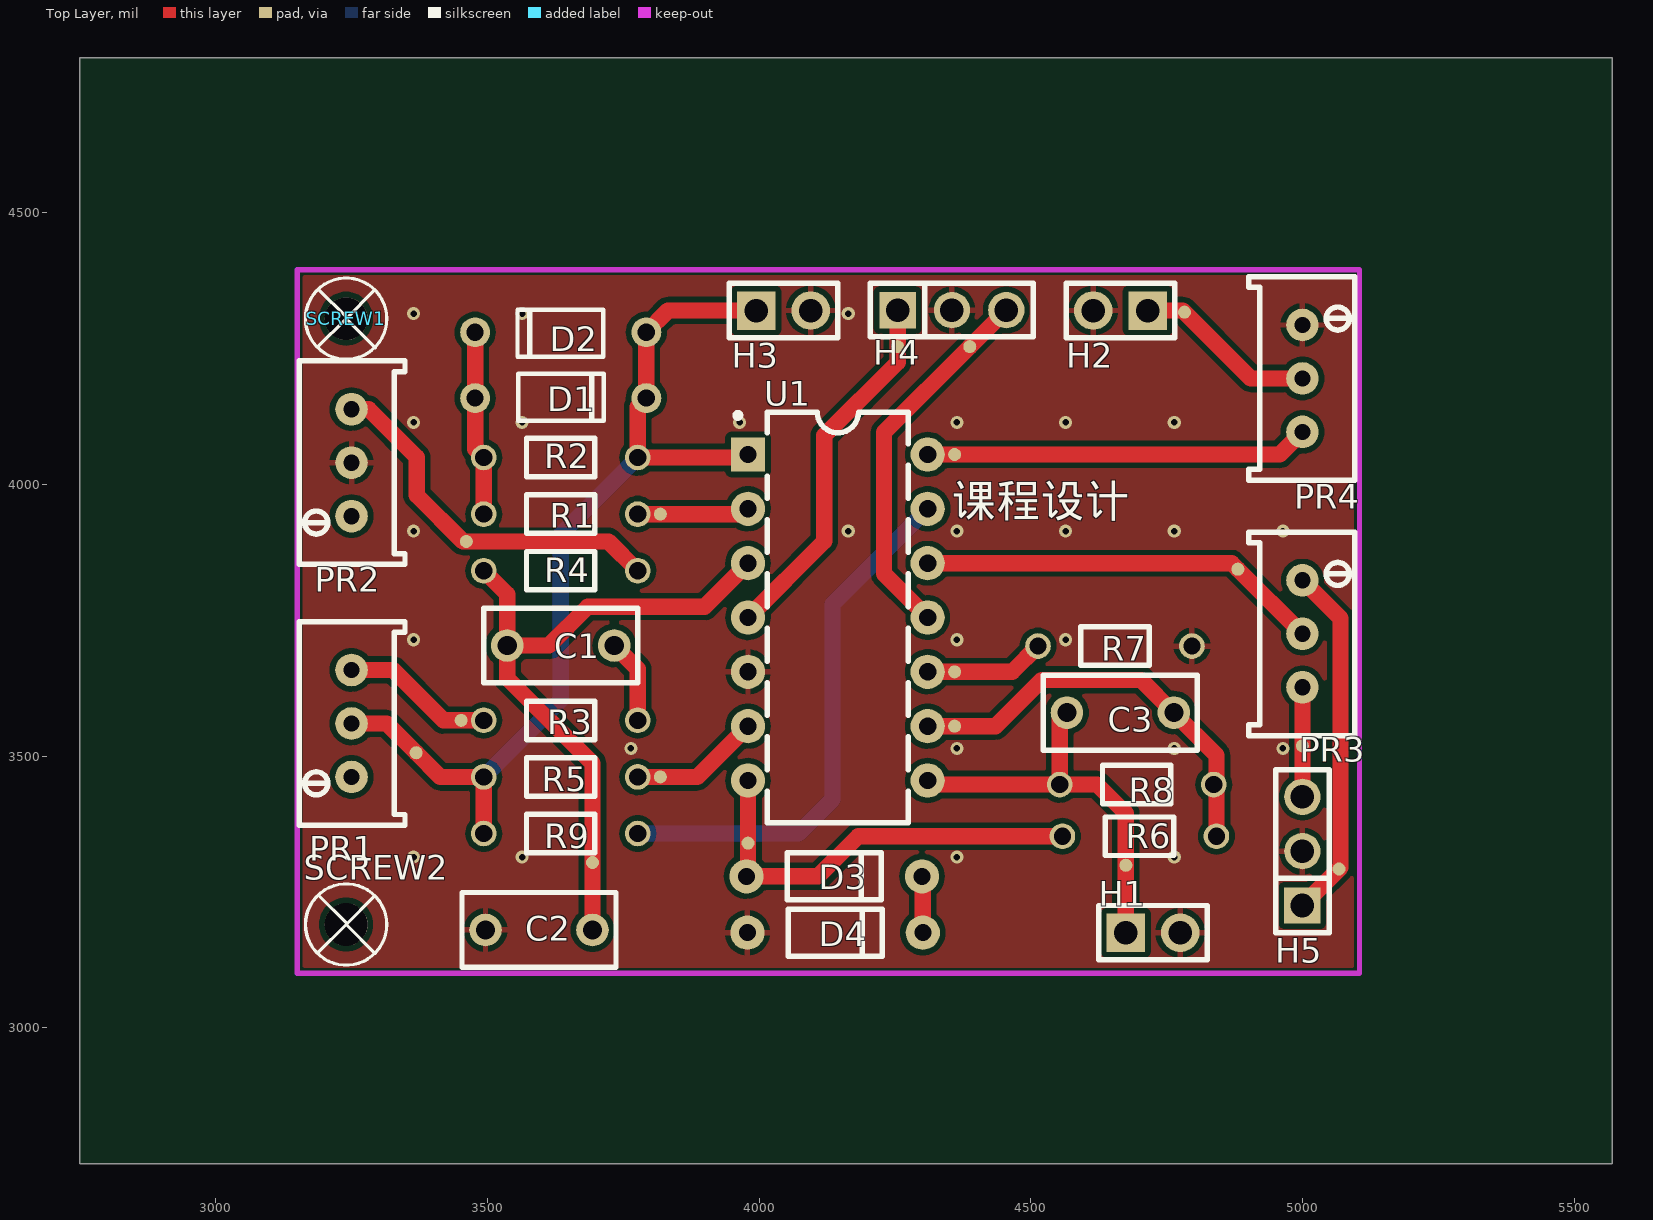
[diagram p0: Top Layer view]
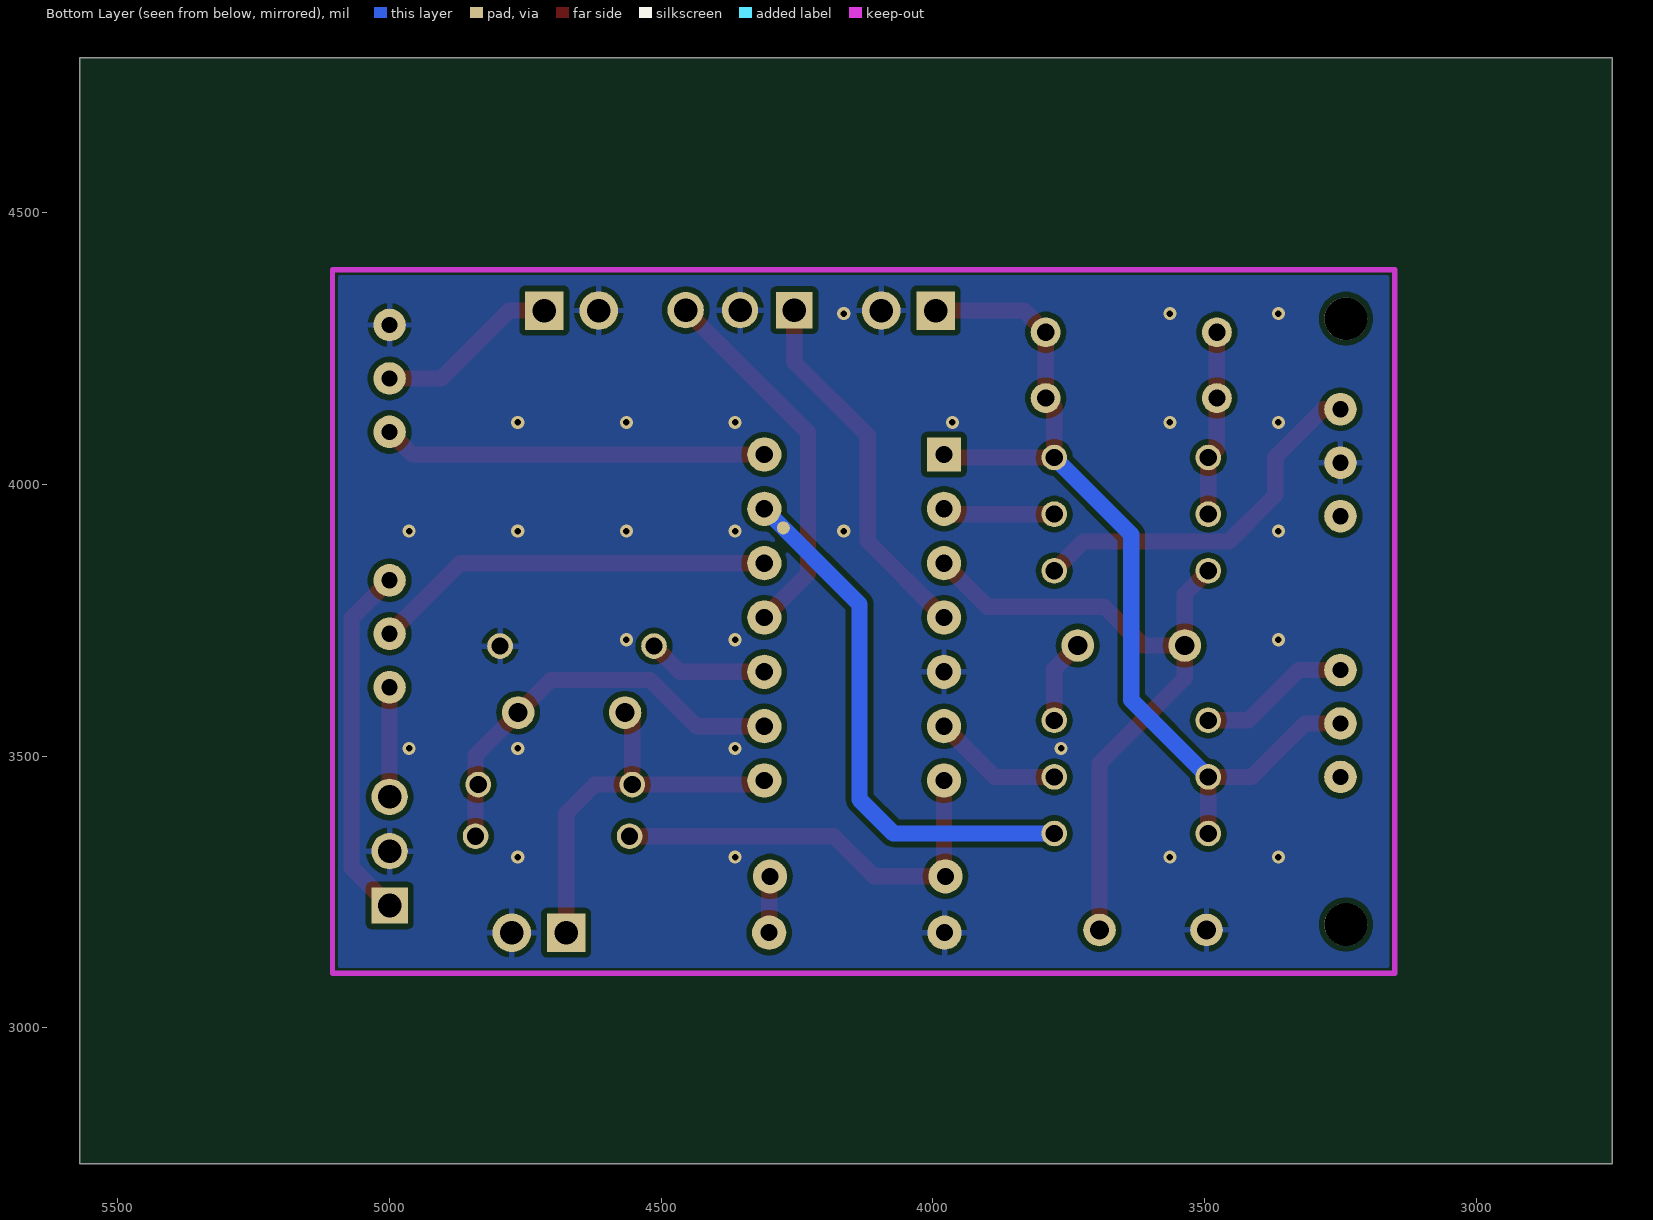
[diagram p1: Bottom Layer view, seen from below]
# Altium PCB MISC51375.pcbdoc
Units mil, origin at the board's own origin, x right, y up, seen from the top; angles counter-clockwise.
Board outline 2820 x 2035 mil, 2 copper layers (Top Layer, Bottom Layer), stack 62.206 mil thick; 28 components, 22 nets, 90 pads, 26 vias.

## Layer stack, top to bottom
Top Solder Mask Layer: solder mask 0.394, Dk 3.3
Top Layer: signal copper 1.379
Dielectric1: surface 59.449, FR4, Dk 4.5
Bottom Layer: signal copper 1.378
Bottom Solder Mask Layer: solder mask 0.394, Dk 3.3

## Board outline
5570,2750 2750,2750 2750,4785 5570,4785

## Design rules (kind name [scope] priority, off if disabled: settings)
BoardOutlineClearance copperThickness2oz_1 [All] p2 off: genericclearance=7.99 ignorepadtopadclearanceinfootprint=FALSE except(0: Arc-SplitContinuation Track-SplitContinuation SMDPad-SplitContinuation THPad-SplitContinuation Via-SplitContinuation Fill-SplitContinuation Region-SplitContinuation Poly-SplitContinuation Text-SplitContinuation Hole-SplitContinuation; 5.98: Arc-CutoutEdge SMDPad-CutoutEdge THPad-CutoutEdge Via-CutoutEdge Fill-CutoutEdge Region-CutoutEdge Text-CutoutEdge; 6.93: Hole-OutlineEdge Hole-CutoutEdge; 10: Poly-OutlineEdge Poly-CutoutEdge; 11.81: Arc-OutlineEdge Track-OutlineEdge SMDPad-OutlineEdge THPad-OutlineEdge Via-OutlineEdge Fill-OutlineEdge Region-OutlineEdge Text-OutlineEdge Track-CutoutEdge)
BoardOutlineClearance copperThickness1oz_1 [All] p4: genericclearance=4.02 ignorepadtopadclearanceinfootprint=FALSE except(0: Arc-SplitContinuation Track-SplitContinuation SMDPad-SplitContinuation THPad-SplitContinuation Via-SplitContinuation Fill-SplitContinuation Region-SplitContinuation Poly-SplitContinuation Text-SplitContinuation Hole-SplitContinuation; 6: SMDPad-CutoutEdge THPad-CutoutEdge Via-CutoutEdge Fill-CutoutEdge Region-CutoutEdge Text-CutoutEdge; 6.93: Hole-OutlineEdge Hole-CutoutEdge; 10: Poly-OutlineEdge Poly-CutoutEdge; 11.8: Arc-OutlineEdge Track-OutlineEdge SMDPad-OutlineEdge THPad-OutlineEdge Via-OutlineEdge Fill-OutlineEdge Region-OutlineEdge Text-OutlineEdge; 11.81: Arc-CutoutEdge Track-CutoutEdge)
Clearance copperThickness2oz [All] p1 off: gap=7.99 ignorepadtopadclearanceinfootprint=FALSE except(5.98: SMDPad-Track SMDPad-SMDPad THPad-Track SMDPad-THPad THPad-THPad Track-Via SMDPad-Via THPad-Via Via-Via Fill-Track Region-Track Fill-SMDPad Region-SMDPad Fill-THPad Region-THPad Fill-Via Region-Via Fill-Fill Fill-Region Region-Region Arc-Track Arc-SMDPad Arc-THPad Arc-Via Fill-Arc Region-Arc Arc-Arc Text-Track SMDPad-Text Text-THPad Text-Via Fill-Text Region-Text Arc-Text Text-Text; 6.93: Hole-Track Hole-SMDPad Hole-THPad Hole-Via Fill-Hole Region-Hole Hole-Arc Hole-Text; 10: Poly-Track Poly-SMDPad Poly-THPad Poly-Via Poly-Fill Poly-Region Poly-Poly Poly-Arc Poly-Text Poly-Hole)
Clearance copperThickness1oz [All] p3: gap=4.02 ignorepadtopadclearanceinfootprint=FALSE except(5.98: SMDPad-Track SMDPad-SMDPad THPad-Track SMDPad-THPad THPad-THPad Track-Via SMDPad-Via THPad-Via Via-Via Fill-Track Region-Track Fill-SMDPad Region-SMDPad Fill-THPad Region-THPad Fill-Via Region-Via Fill-Fill Fill-Region Region-Region; 6: Arc-Track Arc-SMDPad Arc-THPad Arc-Via Fill-Arc Region-Arc Arc-Arc Text-Track SMDPad-Text Text-THPad Text-Via Fill-Text Region-Text Arc-Text Text-Text; 6.93: Hole-Track Hole-SMDPad Hole-THPad Hole-Via Fill-Hole Region-Hole Hole-Arc Hole-Text; 10: Poly-Track Poly-SMDPad Poly-THPad Poly-Via Poly-Fill Poly-Region Poly-Poly Poly-Arc Poly-Text Poly-Hole)
DiffPairsRouting differentialPair [All] p1: maxlimit=6 minlimit=6 mostfreqgap=6 toplayer_minwidth=5 toplayer_prefwidth=10 toplayer_maxwidth=100 toplayer_mingap=6 toplayer_prefgap=6 toplayer_maxgap=6 bottomlayer_minwidth=5 bottomlayer_prefwidth=10 bottomlayer_maxwidth=100 bottomlayer_mingap=6 bottomlayer_prefgap=6 bottomlayer_maxgap=6 maxuncoupledlength=10
HoleToHoleClearance otherClearance [All] p1: gap=11.81 allowstackedmicrovias=TRUE
Length netLength [All] p1: minlimit=0 maxlimit=0
MatchedLengths netLengthTolerance [All] p1: tolerance=1000
PasteMaskExpansion pasteMaskExpansion [All] p1: expansion=0
PlaneConnect innerPlane [All] p1: planeconnectstyle=Relief reliefexpansion=20 reliefentries=4 reliefconductorwidth=10 reliefairgap=10
PolygonConnect copperRegion [(InNet('GND'))] p1: connectstyle=Relief reliefconductorwidth=10 reliefentries=4 polygonreliefangle="90 Angle" airgapwidth=10 via.connectstyle=Relief via.reliefconductorwidth=10 via.reliefentries=4 via.polygonreliefangle="90 Angle" via.airgapwidth=10
RoutingVias viaSize [All] p1: holewidth=12.01 width=24.02 viastyle="Through Hole" minholewidth=11.81 minwidth=19.68 maxholewidth=248.03 maxwidth=393.7
SolderMaskExpansion solderMaskExpansion [IsVia] p1: expansion=-1000 istentingtop=TRUE
SolderMaskExpansion solderMaskExpansion [All] p2: expansion=2 istentingtop=FALSE
Width copperThickness2oz_2 [All] p1 off: maxlimit=100 minlimit=8 preferedwidth=10
Width copperThickness1oz_2 [All] p2: maxlimit=100 minlimit=5 preferedwidth=10

## Components (designator, comment, footprint, x,y, rotation, side; value= is the part's Value field where it differs from the comment)
C1 "10nF" CAP-TH_L7.2-W3.5-P5.00-D0.6 3635.01,3703.46 r0 top
C2 "10nF" CAP-TH_L7.2-W3.5-P5.00-D0.6 3595,3180 r0 top
C3 "10nF" CAP-TH_L7.2-W3.5-P5.00-D0.6 4665,3580 r180 top
D1 "1N4148" DO-35_BD2.2-L4.0-D0.50_1N4148 3635,4158.76 r0 top
D2 "1N4148" DO-35_BD2.2-L4.0-D0.50_1N4148 3635,4280 r180 top
D3 "1.45V" DO-35_BD2.0-L4.2-P8.20-D0.5-RD 4138.43,3278.59 r180 top
D4 "1.45V" DO-35_BD2.0-L4.2-P8.20-D0.5-RD 4140,3175 r180 top
H1 "" HDR-TH_2P-P2.54-V-M-1 4725,3175 r0 top
H2 "" HDR-TH_2P-P2.54-V-M-1 4665,4320 r180 top
H3 "" HDR-TH_2P-P2.54-V-M-1 4045,4320 r0 top
H4 "" HDR-TH_3P-P2.54-V-M 4355,4320.79 r0 top
H5 "" HDR-TH_3P-P2.54-V-M 5000,3325 r90 top
PR1 "100kΩ" R_3296 3245,3560 r90 top
PR2 "100kΩ" R_3296 3245,4040 r90 top
PR3 "1kΩ" R_3296 5005,3725 r270 top
PR4 "1kΩ" R_3296 5005,4195 r270 top
R1 "10kΩ" Res_1/8W 3635,3947.77 r180 top
R2 "10kΩ" Res_1/8W 3635,4046.98 r0 top
R3 "790Ω" Res_1/8W 3635,3568.28 r180 top
R4 "790Ω" Res_1/8W 3635,3838.65 r0 top
R5 "10kΩ" Res_1/8W 3635,3459.16 r0 top
R6 "100kΩ" Res_1/8W 4700,3350 r0 top
R7 "100kΩ" Res_1/8W 4655,3705 r180 top
R8 "1MΩ" Res_1/8W 4695,3450 r180 top
R9 "10kΩ" Res_1/8W 3635,3355 r0 top
SCREW1 "" M2螺丝 3240,4305 r0 top
SCREW2 "" M2螺丝 3240,3190 r0 top
U1 "LM324DT" DIP-14_L19.2-W6.6-P2.54-LS10.9-BL 4145,3755 r270 top

## Footprints (in the part's own frame and the unit in brackets; to place one, negate y for a bottom-side part, rotate by r counter-clockwise, add the part's x,y. Pads: shape width x height; smd on the part's side, far side on the other; paste and mask are expansions set on the pad)
CAP-TH_L7.2-W3.5-P5.00-D0.6 [mil]
  round 60 hole 35.43: 1(-98.43,0) 2(98.42,0)
  silkscreen extent -142,-69 142,69
DIP-14_L19.2-W6.6-P2.54-LS10.9-BL [mil]
  rect 63x63 hole 32: 1(-300,-165.35)
  round 63 hole 32: 2(-200,-165.35) 3(-100,-165.35) 4(0,-165.35) 5(100,-165.35) 6(200,-165.35) 7(300,-165.35) 8(300,165.35) 9(200,165.35) 10(100,165.35) 11(0,165.35) 12(-100,165.35) 13(-200,165.35) 14(-300,165.35)
  silkscreen extent -378,-189 378,130
DO-35_BD2.0-L4.2-P8.20-D0.5-RD [mm]
  round 1.6 hole 0.8: 1(-4.1,0) 2(4.1,0)
  silkscreen extent -2.2,-1.1 2.2,1.1
DO-35_BD2.2-L4.0-D0.50_1N4148 [mm]
  round 1.4 hole 0.8 paste+0 mask+0.05: 1(-4,0) 2(4,0)
  silkscreen extent -1.98,-1.06 2.02,1.14
HDR-TH_2P-P2.54-V-M-1 [mm]
  rect 1.8x1.8 hole 1.1: 1(-1.27,0)
  round 1.8 hole 1.1: 2(1.27,0)
  silkscreen extent -2.54,-1.27 2.54,1.27
HDR-TH_3P-P2.54-V-M [mm]
  rect 1.7x1.7 hole 1.1: 1(-2.54,0)
  round 1.7 hole 1.1: 2(0,0) 3(2.54,0)
  silkscreen extent -3.81,-1.25 3.81,1.25
M2螺丝 [mm]
  round 2 hole 2: 1(0,0)
  silkscreen extent -1.9,-1.9 1.9,1.9
R_3296 [mil]
  round 60 hole 30 paste+0 mask+2: 1(-98.4,-5) 2(0,-5) 3(98.4,-5)
  silkscreen extent -187,-103 187,92
Res_1/8W [mil]
  round 47.2 hole 31.5 paste+0 mask+2: 1(-141.7,2.48) 2(141.7,2.48)
  silkscreen extent -63,-33 63,38

## Free pads (board coordinates)
  round 24 smd: TP1(3693.43,3304.08) TP2(4675,3299.08) TP3(4359.83,3555) TP4(3368.9,3506.1) TP5(3979.65,3339.89) TP6(4783,4317) TP7(3451.72,3565.8) TP8(3461.26,3895) TP9(4881.1,3843.9) TP10(5067.21,3292.21) TP11(5000,3518.8) TP12(4359.83,4055) TP13(3818.28,3945.29) TP14(3818.28,3461.64) TP15(4359.83,3655) TP17(4255,4253.57) TP18(4387.79,4253.57)
  round 24 smd far side: TP16(4275.36,3920.01)

## Via types
v1: diameter 24.02, hole 12, Top Layer to Bottom Layer, 26 vias

## Nets (pads, with @x,y where several pads share a name; then routed paths per layer and width w, separated by ;. In a path a pad name is that pad's centre, name@x,y a point inside that pad or via, vN(x,y) a via of type N, cw(c..) or ccw(c..) an arc to the next point about the centre after c; other vN are vias at no path point)
12V: H4.3 pad.TP18 U1.11 | length 692.3
  Top Layer w30: U1.11 4230,3835.35 4230,4095.79 pad.TP18 H4.3
$1N1: pad.TP13 R1.1 U1.2 | length 207
  Top Layer w30: R1.1 3969.94,3945.29 U1.2
$1N2: D1.1 D2.2 R1.2 R2.1 | length 341.2
  Top Layer w30: D2.2 D1.1 3477.52,4065.23 R2.1 R1.2
$1N6: pad.TP7 PR1.3 R3.2 | length 281.7
  Top Layer w30: PR1.3 3326.6,3658.4 3419.2,3565.8 R3.2
$1N7: C1.2 R3.1 | length 155.6
  Top Layer w30: C1.2 3776.7,3660.19 R3.1
$1N8: C1.1 C2.2 pad.TP1 R4.1 U1.3 | length 1249.9
  Top Layer w30: R4.1 3536.58,3797.85 C1.1 ; C2.2 pad.TP1 3693.43,3486.57 3536.58,3643.42 C1.1 ; U1.3 3899.65,3775 3685,3775 3613.46,3703.46 C1.1
$1N9: pad.TP8 PR2.3 R4.2 | length 690.8
  Top Layer w30: PR2.3 3281.6,4138.4 3370,4050 3370,3980 3455,3895 3722.83,3895 R4.2
$1N11: pad.TP14 R5.2 U1.6 | length 241.6
  Top Layer w30: R5.2 3886.29,3461.64 U1.6
$1N14: C3.1 pad.TP3 R6.2 R8.1 U1.9 | length 773.1
  Top Layer w30: U1.9 4435,3555 4520,3640 4703.43,3640 C3.1 4841.7,3501.72 R6.2
$1N15: D3.2 pad.TP5 R6.1 U1.7 | length 789.4
  Top Layer w30: U1.7 pad.TP5 3979.65,3281.22 D3.2 4108.59,3278.59 4182.48,3352.48 R6.1
$1N16: D3.1 D4.1 | length 104.2
  Top Layer w30: D3.1@4299.85,3278.59 4301.42,3277.02 D4.1
$1N18: pad.TP15 R7.2 U1.10 | length 222.6
  Top Layer w30: U1.10 4465.78,3655 R7.2
$1N20: C3.2 H1.1 pad.TP2 R8.2 U1.8 | length 747.5
  Top Layer w30: U1.8 4317.83,3447.52 R8.2 ; C3.2 4553.3,3566.72 R8.2 ; H1.1 pad.TP2 4675,3395 4622.48,3447.52 R8.2
$1N22: pad.TP16 R9.2 U1.13 | length 991.8
  Bottom Layer w30: R9.2 4072.48,3357.48 4135,3420 4135,3779.65 U1.13
$1N23: D1.2 D2.1 H3.1 pad.TP4 PR1.2 R2.2 R5.1 R9.1 U1.1 | length 1754.8
  Top Layer w30: PR1.2 3315,3560 pad.TP4 3413.36,3461.64 R5.1 R9.1 ; U1.1 3974.1,4049.45 R2.2 3776.7,4142.98 D1.2 D2.1 3832.48,4320 H3.1
  Bottom Layer w30: R5.1 3635,3603.34 3635,3907.75 R2.2
$1N24: pad.TP9 PR3.2 U1.12 | length 743.5
  Top Layer w30: U1.12 4870,3855 pad.TP9 PR3.2
$1N27: pad.TP12 PR4.3 U1.14 | length 706.9
  Top Layer w30: U1.14 4958.4,4055 PR4.3
$1N29: H2.1 pad.TP6 PR4.2 | length 336.8
  Top Layer w30: H2.1 4780,4320 4905,4195 PR4.2
+3V: H5.3 pad.TP11 PR3.3 | length 201.6
  Top Layer w30: H5.3 pad.TP11 PR3.3
-3V: H5.1 pad.TP10 PR3.1 | length 656.4
  Top Layer w30: H5.1 5070,3295 5070,3753.4 PR3.1
-12V: H4.1 pad.TP17 U1.4 | length 679.8
  Top Layer w30: U1.4 4120,3895.35 4120,4090 4255,4225 pad.TP17 H4.1
GND: C2.1 D4.2 H1.2 H2.2 H3.2 H4.2 H5.2 PR2.2 PR4.1 R7.1 U1.5
  other v1: 3364.1,3314.1 3564.1,3314.1 4364.1,3314.1 4764.1,3314.1 3764.1,3514.1 4364.1,3514.1 4764.1,3514.1 4964.1,3514.1 3364.1,3714.1 4364.1,3714.1 4564.1,3714.1 3364.1,3914.1 4164.1,3914.1 4364.1,3914.1 4564.1,3914.1 4764.1,3914.1 4964.1,3914.1 3364.1,4114.1 3564.1,4114.1 3964.1,4114.1 4364.1,4114.1 4564.1,4114.1 4764.1,4114.1 3364.1,4314.1 3564.1,4314.1 4164.1,4314.1
pads on no net: PR1.1 PR2.1 SCREW1.1 SCREW2.1

## Polygon pours and split planes (outlines as drawn)
GND on Top Layer (solid, remove dead copper, pour order 0): 3000,4535 3000,3000 5275,3000 5275,4535
GND on Bottom Layer (solid, remove dead copper, pour order 2): 3035,4475 3035,3000 5320,3000 5320,4475

## Keep-outs
Board Outline Layer:
  lines w10: 3150,3100 3150,4395 5105,4395 5105,3100 3150,3100

## Silkscreen, mask and mechanical layers (free items; w line width, h text height)
Top Silkscreen Layer:
  text "课程设计" at 4355,3940 h60